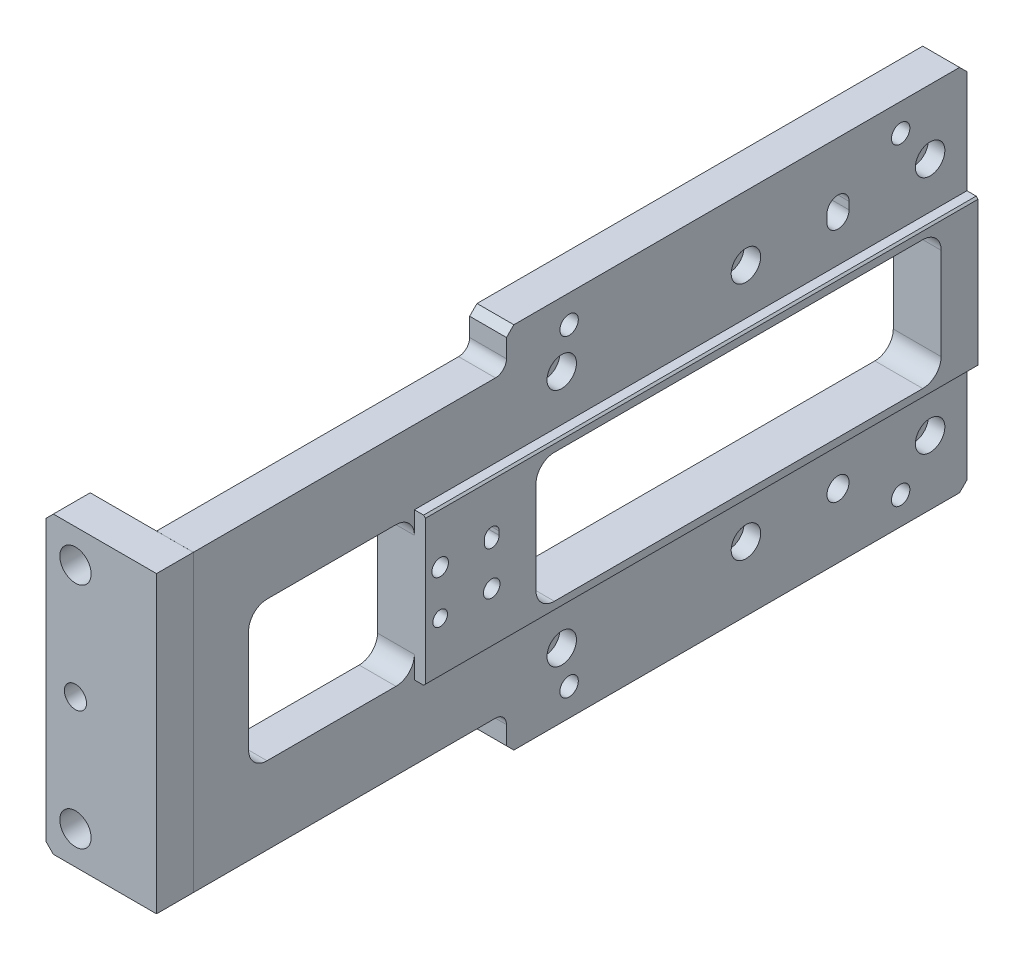
from build123d import *

# Parameters (mm, degrees)
BOSS_EXTRUDE1_DEPTH                                  = 80
CHAMFER1_SIZE                                        = 10
SKETCH2_W                                            = 30
SKETCH2_H                                            = 10
BOSS_EXTRUDE2_DEPTH                                  = 80
SKETCH3_W                                            = 10
SKETCH3_H                                            = 8
CUT_EXTRUDE1_DEPTH                                   = 96
SKETCH4_W                                            = 150
SKETCH4_H                                            = 40
BOSS_EXTRUDE3_DEPTH                                  = 3
CUT_EXTRUDE2_REACH                                   = 236.947
SKETCH5_R                                            = 4.25
CHAMFER5_SIZE                                        = 0.5
SKETCH13_R                                           = 2.25
CUT_EXTRUDE7_DEPTH                                   = 150
SKETCH14_R                                           = 4
CUT_EXTRUDE8_DEPTH                                   = 7.5
SKETCH15_W                                           = 125
SKETCH15_H                                           = 10
BOSS_EXTRUDE5_DEPTH                                  = 10
SKETCH9_R                                            = 1
CUT_EXTRUDE4_DEPTH                                   = 25
M6_TAPPED_HOLE1_D                                    = 5
SKETCH18_W                                           = 45
SKETCH18_H                                           = 38
CUT_EXTRUDE10_DEPTH                                  = 10
FILLET2_R                                            = 5
FILLET3_R                                            = 3
CHAMFER6_SIZE                                        = 2
HOLE_SIZE_PER_SOCKET_HEAD_CAP_SCREW_TYPE_D           = 4.5
HOLE_SIZE_PER_SOCKET_HEAD_CAP_SCREW_TYPE_CBORE_D     = 7.5
HOLE_SIZE_PER_SOCKET_HEAD_CAP_SCREW_TYPE_CBORE_DEPTH = 5
F_4_0_4_DIAMETER_HOLE1_D                             = 4
CUT_EXTRUDE11_DEPTH                                  = 240.977082239
SKETCH24_R                                           = 3
CUT_EXTRUDE12_DEPTH                                  = 239.537208838
SKETCH25_W                                           = 10
SKETCH25_H                                           = 0.01
CUT_EXTRUDE13_DEPTH                                  = 239.537208838
SKETCH26_R                                           = 3
CUT_EXTRUDE14_DEPTH                                  = 230.346898824
CUT_EXTRUDE15_DEPTH                                  = 239.537208838


with BuildPart() as part:
    # Sketch1 → Boss-Extrude1 (new body)
    with BuildSketch(Plane(origin=(0, 0, 0), x_dir=(1, 0, 0), z_dir=(0, 1, 0))):
        Polygon((0, 0), (20, 0), (20, 8), (10, 8), (10, 220), (0, 220), align=None)
    extrude(amount=BOSS_EXTRUDE1_DEPTH)

    # Chamfer1
    chamfer1_edges = [part.edges().sort_by_distance(p)[0] for p in [
        (20, 80, -4),
        (20, 0, -4),
    ]]
    chamfer(chamfer1_edges, length=CHAMFER1_SIZE)

    # Sketch2 → Boss-Extrude2 (add)
    with BuildSketch(Plane.XZ):
        with Locations((-5, -5)):
            Rectangle(SKETCH2_W, SKETCH2_H)
    extrude(amount=-BOSS_EXTRUDE2_DEPTH)

    # Sketch3 → Cut-Extrude1 (cut)
    with BuildSketch(Plane.XZ):
        with Locations((15, -4)):
            Rectangle(SKETCH3_W, SKETCH3_H)
    extrude(amount=-CUT_EXTRUDE1_DEPTH, mode=Mode.SUBTRACT)

    # Sketch4 → Boss-Extrude3 (add)
    with BuildSketch(Plane(origin=(10, 0, 0), x_dir=(0, 0, -1), z_dir=(1, 0, 0))):
        with Locations((145, 40)):
            Rectangle(SKETCH4_W, SKETCH4_H)
    extrude(amount=BOSS_EXTRUDE3_DEPTH)

    # Sketch5 → Cut-Extrude2 (cut, up to next)
    with BuildSketch(Plane(origin=(0, 0, 0), x_dir=(-1, 0, 0), z_dir=(0, 0, -1)), mode=Mode.PRIVATE) as cut_extrude2_sk1:
        with Locations((12, 71)):
            Circle(SKETCH5_R)
    cut_extrude2_tool1 = extrude(cut_extrude2_sk1.sketch, amount=CUT_EXTRUDE2_REACH, mode=Mode.PRIVATE) & part.part
    # Sketch5 → Cut-Extrude2 (cut, up to next)
    with BuildSketch(Plane(origin=(0, 0, 0), x_dir=(-1, 0, 0), z_dir=(0, 0, -1)), mode=Mode.PRIVATE) as cut_extrude2_sk2:
        with Locations(Location((12, 9, 0), (0, 0, 180))):
            Circle(SKETCH5_R)
    cut_extrude2_tool2 = extrude(cut_extrude2_sk2.sketch, amount=CUT_EXTRUDE2_REACH, mode=Mode.PRIVATE) & part.part
    add(cut_extrude2_tool1.solids().sort_by_distance((-12, 71, 0))[0], mode=Mode.SUBTRACT)
    add(cut_extrude2_tool2.solids().sort_by_distance((-12, 9, 0))[0], mode=Mode.SUBTRACT)

    # Chamfer5
    chamfer5_edges = [part.edges().sort_by_distance(p)[0] for p in [
        (13, 60, -145),
        (13, 20, -145),
    ]]
    chamfer(chamfer5_edges, length=CHAMFER5_SIZE)

    # Sketch13 → Cut-Extrude7 (cut)
    with BuildSketch(Plane(origin=(13, 0, 0), x_dir=(0, 0, -1), z_dir=(1, 0, 0))):
        with Locations((210, 72.5)):
            Circle(SKETCH13_R)
        with Locations((110, 72.5)):
            Circle(SKETCH13_R)
        with Locations((210, 7.5)):
            Circle(SKETCH13_R)
        with Locations((110, 7.5)):
            Circle(SKETCH13_R)
        with Locations((160, 72.5)):
            Circle(SKETCH13_R)
        with Locations((160, 7.5)):
            Circle(SKETCH13_R)
    extrude(amount=-CUT_EXTRUDE7_DEPTH, mode=Mode.SUBTRACT)

    # Sketch14 → Cut-Extrude8 (cut)
    with BuildSketch(Plane(origin=(13, 0, 0), x_dir=(0, 0, -1), z_dir=(1, 0, 0))):
        with Locations((110, 72.5)):
            Circle(SKETCH14_R)
        with Locations((110, 7.5)):
            Circle(SKETCH14_R)
        with Locations((210, 7.5)):
            Circle(SKETCH14_R)
        with Locations((210, 72.5)):
            Circle(SKETCH14_R)
        with Locations((160, 72.5)):
            Circle(SKETCH14_R)
        with Locations((160, 7.5)):
            Circle(SKETCH14_R)
    extrude(amount=-CUT_EXTRUDE8_DEPTH, mode=Mode.SUBTRACT)

    # Sketch15 → Boss-Extrude5 (add)
    with BuildSketch(Plane.ZY):
        with Locations((-157.5, -5)):
            Rectangle(SKETCH15_W, SKETCH15_H)
        with Locations((-157.5, 85)):
            Rectangle(SKETCH15_W, SKETCH15_H)
    extrude(amount=-BOSS_EXTRUDE5_DEPTH)

    # Sketch9 → Cut-Extrude4 (cut)
    with BuildSketch(Plane(origin=(10, 0, 0), x_dir=(0, 0, -1), z_dir=(1, 0, 0))):
        with Locations((202, 82.5)):
            Circle(SKETCH9_R)
        with Locations((112, 82.5)):
            Circle(SKETCH9_R)
        with Locations((112, -2.5)):
            Circle(SKETCH9_R)
        with Locations((202, -2.5)):
            Circle(SKETCH9_R)
    extrude(amount=-CUT_EXTRUDE4_DEPTH, mode=Mode.SUBTRACT)

    # M6 Tapped Hole1 (through all)
    with Locations(Plane(origin=(10, 82.5, -202), x_dir=(0, 0, 1), z_dir=(1, 0, 0))):
        with Locations((0, 0), (90, 0), (90, 85), (0, 85)):
            Hole(M6_TAPPED_HOLE1_D / 2)

    # Sketch18 → Cut-Extrude10 (cut)
    with BuildSketch(Plane(origin=(10, 0, 0), x_dir=(0, 0, -1), z_dir=(1, 0, 0))):
        with Locations((47.5, 40)):
            Rectangle(SKETCH18_W, SKETCH18_H)
    extrude(amount=-CUT_EXTRUDE10_DEPTH, mode=Mode.SUBTRACT)

    # Fillet2
    fillet2_edges = [part.edges().sort_by_distance(p)[0] for p in [
        (5, 59, -70),
        (5, 21, -70),
        (5, 21, -25),
        (5, 59, -25),
    ]]
    fillet(fillet2_edges, radius=FILLET2_R)

    # Fillet3
    fillet3_edges = [part.edges().sort_by_distance(p)[0] for p in [
        (5, 80, -95),
        (5, 0, -95),
    ]]
    fillet(fillet3_edges, radius=FILLET3_R)

    # Chamfer6
    chamfer6_edges = [part.edges().sort_by_distance(p)[0] for p in [
        (5, 90, -220),
        (5, -10, -220),
        (5, 90, -95),
        (5, -10, -95),
        (-20, 80, -5),
        (-20, 0, -5),
    ]]
    chamfer(chamfer6_edges, length=CHAMFER6_SIZE)

    # Hole size per socket head cap screw type 5 (through all)
    with Locations(Plane.ZY):
        with Locations((-88, 34), (-74, 46)):
            CounterBoreHole(HOLE_SIZE_PER_SOCKET_HEAD_CAP_SCREW_TYPE_D / 2, HOLE_SIZE_PER_SOCKET_HEAD_CAP_SCREW_TYPE_CBORE_D / 2, HOLE_SIZE_PER_SOCKET_HEAD_CAP_SCREW_TYPE_CBORE_DEPTH)

    # Ø4.0 (4) Diameter Hole1 (through all)
    with Locations(Plane.ZY):
        with Locations((-74, 34), (-88, 46)):
            Hole(F_4_0_4_DIAMETER_HOLE1_D / 2)

    # Sketch23 → Cut-Extrude11 (cut, through all)
    with BuildSketch(Plane(origin=(13, 0, 0), x_dir=(0, 0, -1), z_dir=(1, 0, 0))):
        with BuildLine():
            Line((105, 57.5), (205, 57.5))
            ThreePointArc((205, 57.5), (208.535533906, 56.035533906), (210, 52.5))
            Line((210, 52.5), (210, 27.5))
            ThreePointArc((210, 27.5), (208.535533906, 23.964466094), (205, 22.5))
            Line((205, 22.5), (105, 22.5))
            ThreePointArc((105, 22.5), (101.464466094, 23.964466094), (100, 27.5))
            Line((100, 27.5), (100, 52.5))
            ThreePointArc((100, 52.5), (101.464466094, 56.035533906), (105, 57.5))
        make_face()
    extrude(amount=-CUT_EXTRUDE11_DEPTH, mode=Mode.SUBTRACT)

    # Sketch24 → Cut-Extrude12 (cut, through all)
    with BuildSketch(Plane.ZY):
        with Locations((-185, 7.5)):
            Circle(SKETCH24_R)
        with BuildLine():
            Line((-188, 71.5), (-188, 73.5))
            ThreePointArc((-188, 73.5), (-185, 76.5), (-182, 73.5))
            Line((-182, 73.5), (-182, 71.5))
            ThreePointArc((-182, 71.5), (-185, 68.5), (-188, 71.5))
        make_face()
    extrude(amount=-CUT_EXTRUDE12_DEPTH, mode=Mode.SUBTRACT)

    # Sketch25 → Cut-Extrude13 (cut, through all)
    with BuildSketch(Plane.XZ):
        with Locations((5, -10.005)):
            Rectangle(SKETCH25_W, SKETCH25_H)
    extrude(amount=-CUT_EXTRUDE13_DEPTH, mode=Mode.SUBTRACT)


with BuildPart() as cut_extrude13_piece_1:
    # of the separate pieces the step leaves, piece 1, a body of its own (cut_extrude13_pieces)
    add(part.part.solids().sort_by_distance((10, -8, -95))[0])

    # Sketch28 → Cut-Extrude15 (cut, through all)
    with BuildSketch(Plane.ZY):
        with BuildLine():
            Line((-86, 46.5), (-86, 45.5))
            ThreePointArc((-86, 45.5), (-88, 43.5), (-90, 45.5))
            Line((-90, 45.5), (-90, 46.5))
            ThreePointArc((-90, 46.5), (-88, 48.5), (-86, 46.5))
        make_face()
    extrude(amount=-CUT_EXTRUDE15_DEPTH, mode=Mode.SUBTRACT)


with BuildPart() as cut_extrude13_piece_2:
    # of the separate pieces the step leaves, piece 2, a body of its own (cut_extrude13_pieces)
    add(part.part.solids().sort_by_distance((10, 0, -10))[0])

    # Sketch26 → Cut-Extrude14 (cut, through all)
    with BuildSketch(Plane(origin=(0, 0, -10), x_dir=(-1, 0, 0), z_dir=(0, 0, -1))):
        with Locations((12, 40)):
            Circle(SKETCH26_R)
    extrude(amount=-CUT_EXTRUDE14_DEPTH, mode=Mode.SUBTRACT)


solid = Compound([cut_extrude13_piece_1.part, cut_extrude13_piece_2.part])
